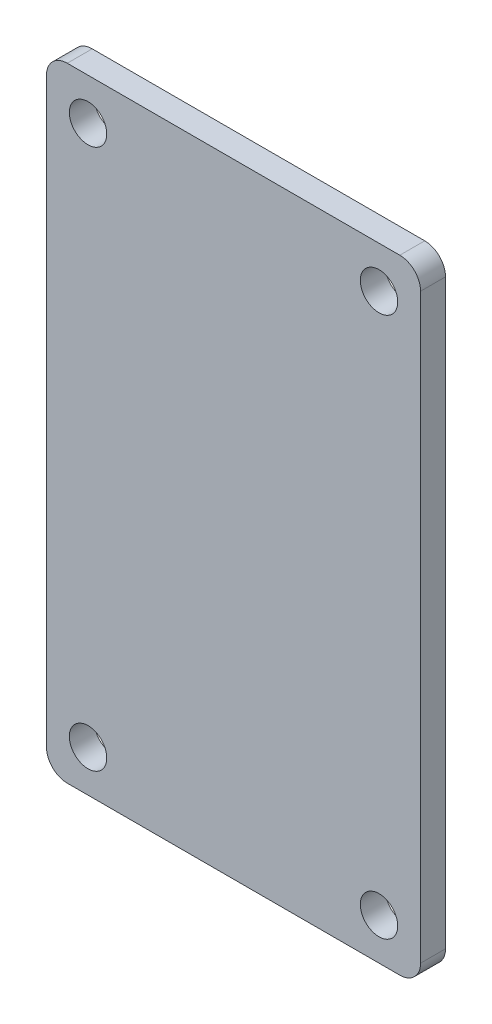
SolidWorks part; units mm, degrees
material "普通碳钢"
ref_plane "Front Plane" through (0, 0, 0) normal (0, 0, 1) x (1, 0, 0)
ref_plane "Top Plane" through (0, 0, 0) normal (0, 1, 0) x (1, 0, 0)
ref_plane "Right Plane" through (0, 0, 0) normal (1, 0, 0) x (0, 0, -1)
sketch "Sketch1" plane through (0, 0, 0) normal (0, 0, 1) x (1, 0, 0)
  line L2 (80, 150) -> (-80, 150)
  line L3 (-90, 140) -> (-90, -140)
  line L4 (-80, -150) -> (80, -150)
  line L5 (90, -140) -> (90, 140)
  arc A0 (-80, 150) -> (-90, 140) centre (-80, 140) ccw
  arc A1 (90, 140) -> (80, 150) centre (80, 140) ccw
  arc A2 (80, -150) -> (90, -140) centre (80, -140) ccw
  arc A3 (-90, -140) -> (-80, -150) centre (-80, -140) ccw
  point P3 (-90, 150)
  point P12 (90, -150)
  point P15 (-90, -150)
  dimension "D3" = 10
  dimension "D1" = 180
  dimension "D2" = 300
extrude "Extrude1" add sketch "Sketch1" along normal mid plane 12
sketch "Sketch2" plane through (0, 0, 6) normal (0, 0, 1) x (1, 0, 0)
  line L0 (-90, 140) -> (-90, -140) construction
  line L1 (-80, -150) -> (80, -150) construction
  line L2 (-70, -130) -> (70, -130) construction
  line L3 (-70, -130) -> (-70, 130) construction
  circle A0 centre (-70, -130) radius 9
  circle A1 centre (70, -130) radius 9
  circle A2 centre (-70, 130) radius 9
  circle A3 centre (70, 130) radius 9
  dimension "D3" = 18
  dimension "D1" = 20
  dimension "D2" = 20
  dimension "D4" = 140
  dimension "D5" = 260
extrude "Extrude2" cut sketch "Sketch2" against normal through all
